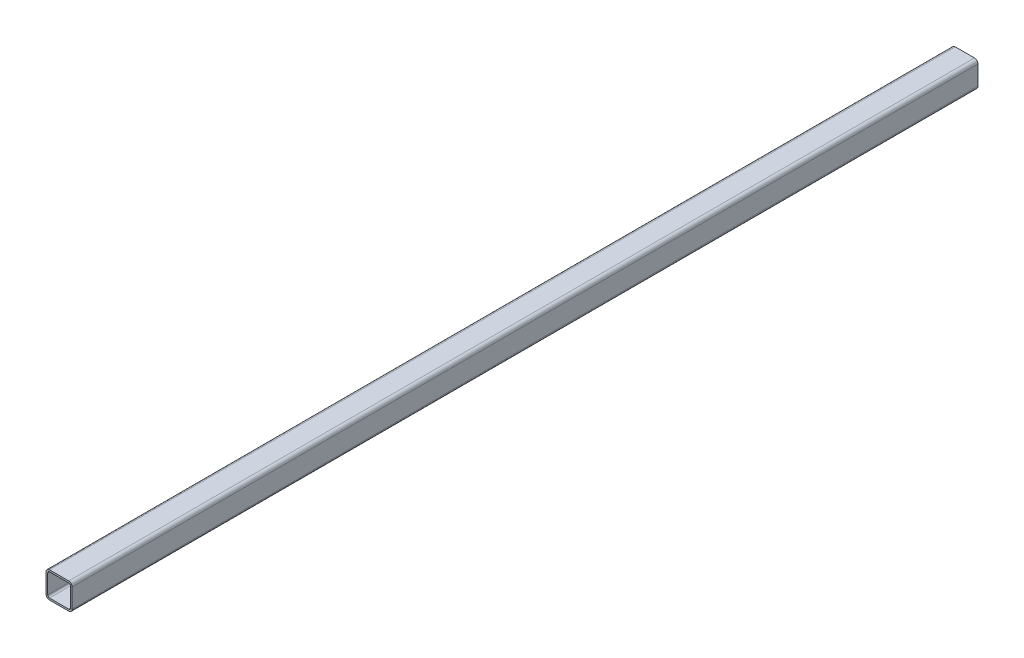
from build123d import *

# Parameters (mm, degrees)
EXTRUDE_THIN1_DEPTH = 518.8


with BuildPart() as part:
    # Sketch1 → Extrude-Thin1 (new, symmetric)
    with BuildSketch(Plane.XY):
        with BuildLine():
            Line((-15, 11), (-15, -11))
            ThreePointArc((-15, -11), (-13.828427125, -13.828427125), (-11, -15))
            Line((-11, -15), (11, -15))
            ThreePointArc((11, -15), (13.828427125, -13.828427125), (15, -11))
            Line((15, -11), (15, 11))
            ThreePointArc((15, 11), (13.828427125, 13.828427125), (11, 15))
            Line((11, 15), (-11, 15))
            ThreePointArc((-11, 15), (-13.828427125, 13.828427125), (-15, 11))
        make_face()
        with BuildLine():
            Line((-13, 11), (-13, -11))
            ThreePointArc((-13, -11), (-12.414213562, -12.414213562), (-11, -13))
            Line((-11, -13), (11, -13))
            ThreePointArc((11, -13), (12.414213562, -12.414213562), (13, -11))
            Line((13, -11), (13, 11))
            ThreePointArc((13, 11), (12.414213562, 12.414213562), (11, 13))
            Line((11, 13), (-11, 13))
            ThreePointArc((-11, 13), (-12.414213562, 12.414213562), (-13, 11))
        make_face(mode=Mode.SUBTRACT)
    extrude(amount=EXTRUDE_THIN1_DEPTH, both=True)


solid = part.part
